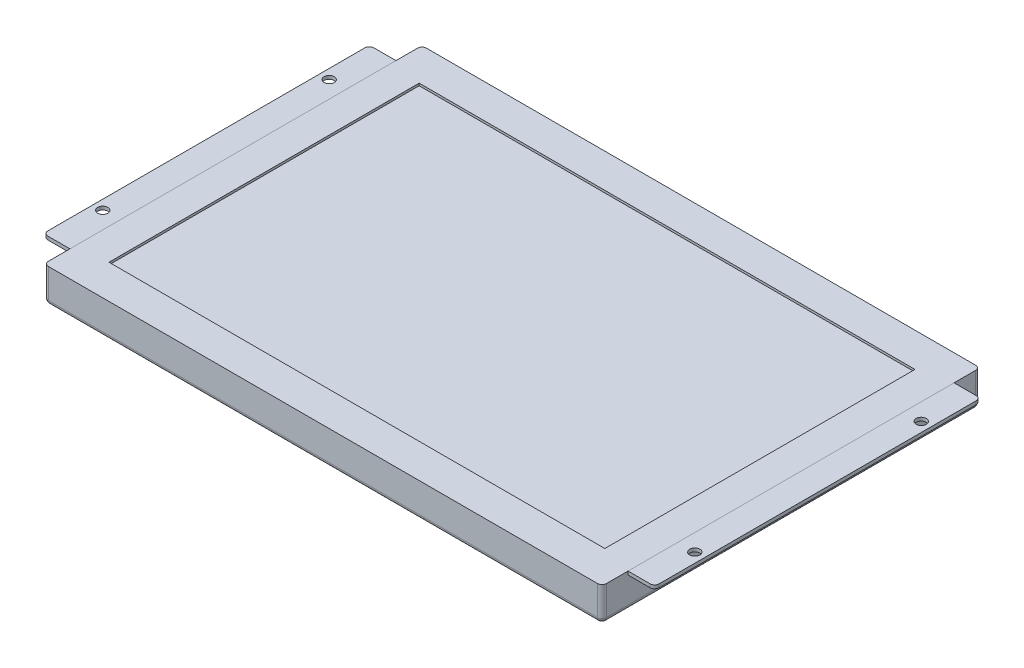
from build123d import *

# Parameters (mm, degrees)
SKETCH_1_W                       = 246.5
SKETCH_1_H                       = 167
EXTRUDE_1_DEPTH                  = 15
SKETCH_3_W                       = 160
SKETCH_3_H                       = 94
EXTRUDE_2_DEPTH                  = 20
FILLET_1_R                       = 2
SKETCH_4_W                       = 219
SKETCH_4_H                       = 137
CUT_EXTRUDE_1_DEPTH              = 1
SKETCH_5_W                       = 11.75
SKETCH_5_H                       = 144
EXTRUDE_3_DEPTH                  = 1.5
EXTRUDE_3_2_DEPTH                = 1.5
SKETCH_6_W                       = 2.25
SKETCH_6_H                       = 35
HOLE_WIZARD_4_5_4_5_1_AT_2_COUNT = 2
HOLE_WIZARD_4_5_4_5_1_AT_2_PITCH = 100
HOLE_WIZARD_4_5_4_5_1_AT_3_COUNT = 2
HOLE_WIZARD_4_5_4_5_1_AT_3_PITCH = 279.968301777
HOLE_WIZARD_4_5_4_5_1_AT_4_COUNT = 2
HOLE_WIZARD_4_5_4_5_1_AT_4_PITCH = 261.5
FILLET_2_R                       = 2
FILLET_3_R                       = 2


with BuildPart() as part:
    # 草图1 → 凸台-拉伸1 (new body)
    with BuildSketch(Plane(origin=(0, 0, 0), x_dir=(1, 0, 0), z_dir=(0, 1, 0))):
        Rectangle(SKETCH_1_W, SKETCH_1_H)
    extrude(amount=EXTRUDE_1_DEPTH)

    # 草图3 → 凸台-拉伸2 (add)
    with BuildSketch(Plane.XZ):
        Rectangle(SKETCH_3_W, SKETCH_3_H)
    extrude(amount=EXTRUDE_2_DEPTH)

    # 圆角1
    fillet_1_edges = [part.edges().sort_by_distance(p)[0] for p in [
        (-80, 0, 0),
        (-80, -10, 47),
        (0, 0, -47),
        (-80, -10, -47),
        (80, 0, 0),
        (80, -10, -47),
        (0, 0, 47),
        (80, -10, 47),
        (-80, -20, 0),
        (0, -20, -47),
        (80, -20, 0),
        (0, -20, 47),
        (0, 0, 83.5),
        (-123.25, 0, 0),
        (0, 0, -83.5),
        (123.25, 0, 0),
        (123.25, 7.5, 83.5),
        (-123.25, 7.5, 83.5),
        (-123.25, 7.5, -83.5),
        (123.25, 7.5, -83.5),
    ]]
    fillet(fillet_1_edges, radius=FILLET_1_R)

    # 草图4 → 切除-拉伸1 (cut)
    with BuildSketch(Plane(origin=(0, 15, 0), x_dir=(1, 0, 0), z_dir=(0, 1, 0))):
        Rectangle(SKETCH_4_W, SKETCH_4_H)
    extrude(amount=-CUT_EXTRUDE_1_DEPTH, mode=Mode.SUBTRACT)


with BuildPart() as body_2:
    # 草图5 → 凸台-拉伸3 (new body)
    with BuildSketch(Plane(origin=(0, 15, 0), x_dir=(1, 0, 0), z_dir=(0, 1, 0))):
        with Locations((129.125, 0)):
            Rectangle(SKETCH_5_W, SKETCH_5_H)
    extrude(amount=-EXTRUDE_3_DEPTH)

    # 草图6 → Ø4.5 (4.5) 直径孔1 (revolve, cut)
    with BuildSketch(Plane(origin=(130.75, 15, -50), x_dir=(0, 0, 1), z_dir=(1, 0, 0))):
        with Locations((1.125, 17.5)):
            Rectangle(SKETCH_6_W, SKETCH_6_H)
    hole_wizard_4_5_4_5_1 = revolve(axis=Axis((130.75, 21.35, -50), (0, -1, 0)), mode=Mode.SUBTRACT)

    # Ø4.5 (4.5) 直径孔1 at 2: Ø4.5 (4.5) 直径孔1 ×2
    with Locations(*[(0, 0, i * HOLE_WIZARD_4_5_4_5_1_AT_2_PITCH) for i in range(1, HOLE_WIZARD_4_5_4_5_1_AT_2_COUNT)]):
        add(hole_wizard_4_5_4_5_1, mode=Mode.SUBTRACT)

    # 圆角2
    fillet_2_edges = [body_2.edges().sort_by_distance(p)[0] for p in [
        (135, 14.25, -72),
        (135, 14.25, 72),
    ]]
    fillet(fillet_2_edges, radius=FILLET_2_R)


with BuildPart() as body_3:
    # 草图5 → Extrude 3 2 (new body)
    with BuildSketch(Plane(origin=(0, 15, 0), x_dir=(1, 0, 0), z_dir=(0, 1, 0))):
        with Locations((-129.125, 0)):
            Rectangle(SKETCH_5_W, SKETCH_5_H)
    extrude(amount=-EXTRUDE_3_2_DEPTH)

    # Ø4.5 (4.5) 直径孔1 at 3: Ø4.5 (4.5) 直径孔1 ×2
    with Locations(*[Vector(-0.9340343115275901, 0, 0.35718329312718555) * (i * HOLE_WIZARD_4_5_4_5_1_AT_3_PITCH) for i in range(1, HOLE_WIZARD_4_5_4_5_1_AT_3_COUNT)]):
        add(hole_wizard_4_5_4_5_1, mode=Mode.SUBTRACT)

    # Ø4.5 (4.5) 直径孔1 at 4: Ø4.5 (4.5) 直径孔1 ×2
    with Locations(*[(-i * HOLE_WIZARD_4_5_4_5_1_AT_4_PITCH, 0, 0) for i in range(1, HOLE_WIZARD_4_5_4_5_1_AT_4_COUNT)]):
        add(hole_wizard_4_5_4_5_1, mode=Mode.SUBTRACT)

    # 圆角3
    fillet_3_edges = [body_3.edges().sort_by_distance(p)[0] for p in [
        (-135, 14.25, -72),
        (-135, 14.25, 72),
    ]]
    fillet(fillet_3_edges, radius=FILLET_3_R)


solid = Compound([part.part, body_2.part, body_3.part])
